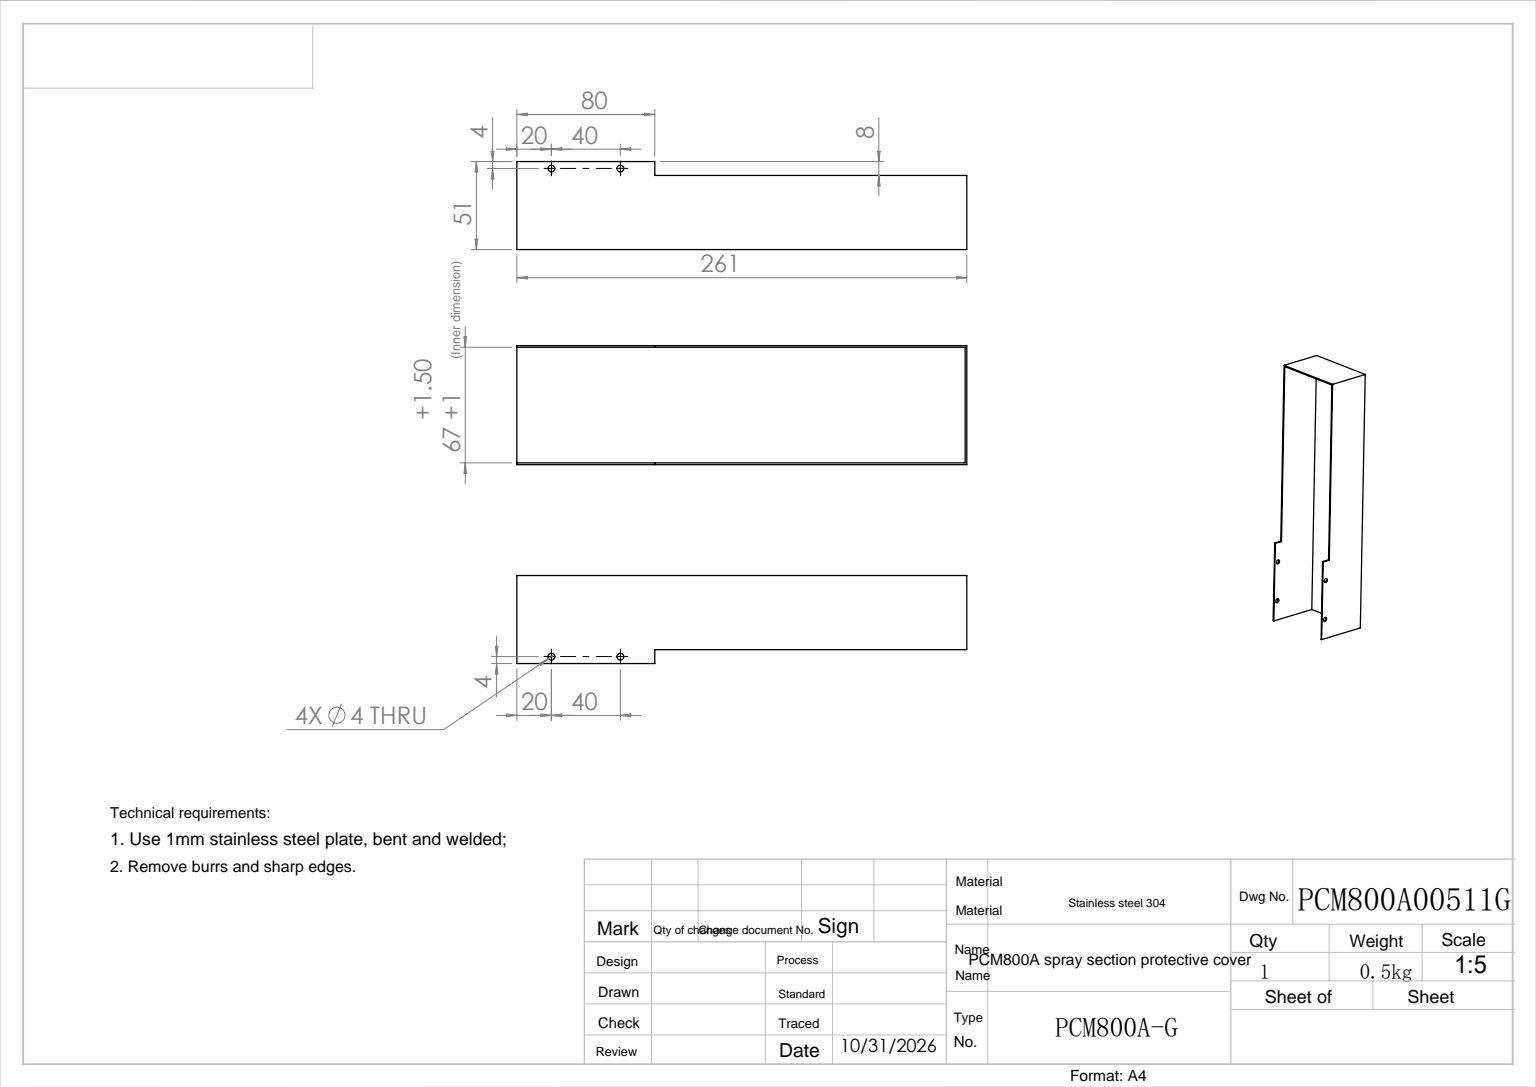
SolidWorks part; units mm, degrees
ref_plane "前视基准面" through (0, 0, 0) normal (0, 0, 1) x (1, 0, 0)
ref_plane "上视基准面" through (0, 0, 0) normal (0, 1, 0) x (1, 0, 0)
ref_plane "右视基准面" through (0, 0, 0) normal (1, 0, 0) x (0, 0, -1)
sketch "草图1" plane through (0, 0, 0) normal (0, 0, 1) x (1, 0, 0)
  line L0 (5.1231, -134.9499) -> (5.1231, -314.9499)
  line L1 (5.1231, -134.9499) -> (47.1231, -134.9499)
  line L2 (-2.8769, -314.9499) -> (-2.8769, -394.9499)
  line L3 (-2.8769, -394.9499) -> (47.1231, -394.9499)
  line L4 (47.1231, -134.9499) -> (47.1231, -394.9499)
  line L5 (5.1231, -314.9499) -> (-2.8769, -314.9499)
  dimension "D1" = 260
  dimension "D2" = 180
  dimension "D3" = 50
  dimension "D4" = 8
extrude "凸台-拉伸1" add sketch "草图1" along normal blind 67
shell "抽壳1" thickness 1
sketch "草图2" plane through (0, 0, 68) normal (0, 0, 1) x (1, 0, 0)
  line L0 (-2.8769, -394.9499) -> (48.1231, -394.9499) construction
  line L1 (-2.8769, -314.9499) -> (-2.8769, -394.9499) construction
  circle A0 centre (1.1231, -374.9499) radius 2
  dimension "D1" = 4
  dimension "D2" = 20
  dimension "D3" = 4
extrude "切除-拉伸1" cut sketch "草图2" against normal through all
pattern_linear "阵列(线性)1" count 2 spacing 40 along (0, 1, 0) of "切除-拉伸1"
